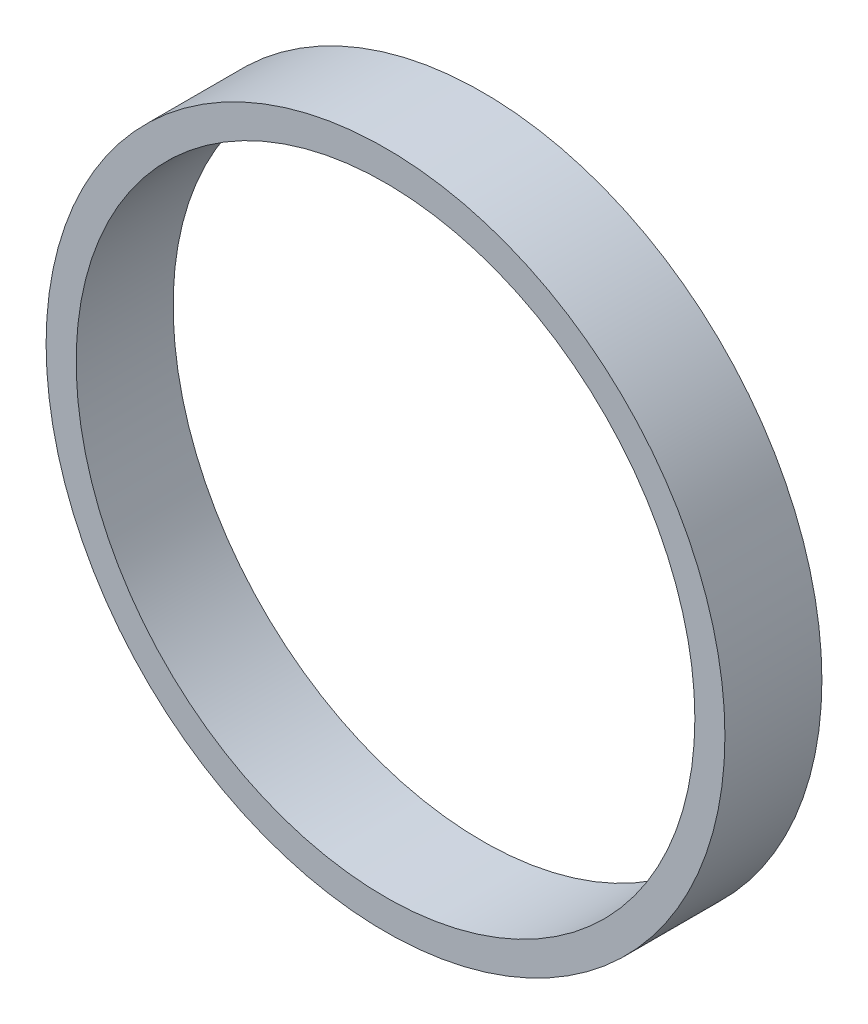
from build123d import *

# Parameters (mm, degrees)
SKETCH1_R           = 175
SKETCH1_R_2         = 159.5
BOSS_EXTRUDE1_DEPTH = 25


with BuildPart() as part:
    # Sketch1 → Boss-Extrude1 (new, symmetric)
    with BuildSketch(Plane.XY):
        Circle(SKETCH1_R)
        Circle(SKETCH1_R_2, mode=Mode.SUBTRACT)
    extrude(amount=BOSS_EXTRUDE1_DEPTH, both=True)


solid = part.part
